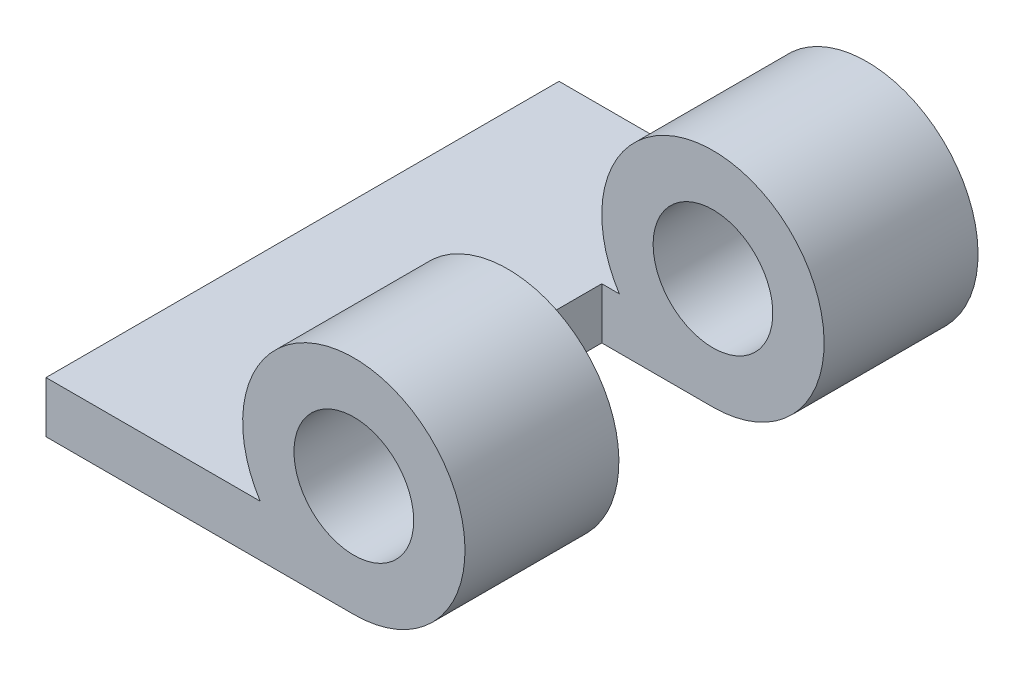
SolidWorks part; units mm, degrees
ref_plane "前视基准面" through (0, 0, 0) normal (0, 0, 1) x (1, 0, 0)
ref_plane "上视基准面" through (0, 0, 0) normal (0, 1, 0) x (1, 0, 0)
ref_plane "右视基准面" through (0, 0, 0) normal (1, 0, 0) x (0, 0, -1)
sketch "草图1" plane through (0, 0, 0) normal (0, 0, 1) x (1, 0, 0)
  line L1 (-9, 1.5) -> (3.5228, 1.5)
  line L2 (-9, 1.5) -> (-9, -1.5)
  line L3 (-9, -1.5) -> (9, -1.5)
  line L5 (-9, 1.5) -> (9, -1.5) construction
  line L6 (-9, -1.5) -> (9, 1.5) construction
  arc A0 (9, -1.5) -> (3.5228, 1.5) centre (9, 5) ccw
  circle A1 centre (9, 5) radius 3.5
  circle A2 centre (9, 5) radius 6.5 construction
  point P0 (0, 0)
  dimension "D3" = 13
  dimension "D1" = 3
  dimension "D2" = 18
  dimension "D4" = 3
extrude "凸台-拉伸1" add sketch "草图1" along normal blind 30
sketch "草图2" plane through (0, 0, 0) normal (0, 1, 0) x (1, 0, 0)
  line L0 (2.5, 0) -> (2.5, -30) construction
  line L1 (2.5, -9) -> (21.833, -9)
  line L2 (2.5, -9) -> (2.5, -21)
  line L3 (2.5, -21) -> (21.833, -21)
  line L4 (21.833, -9) -> (21.833, -21)
  dimension "D1" = 9
  dimension "D2" = 9
extrude "切除-拉伸1" cut sketch "草图2" against normal mid plane 30
